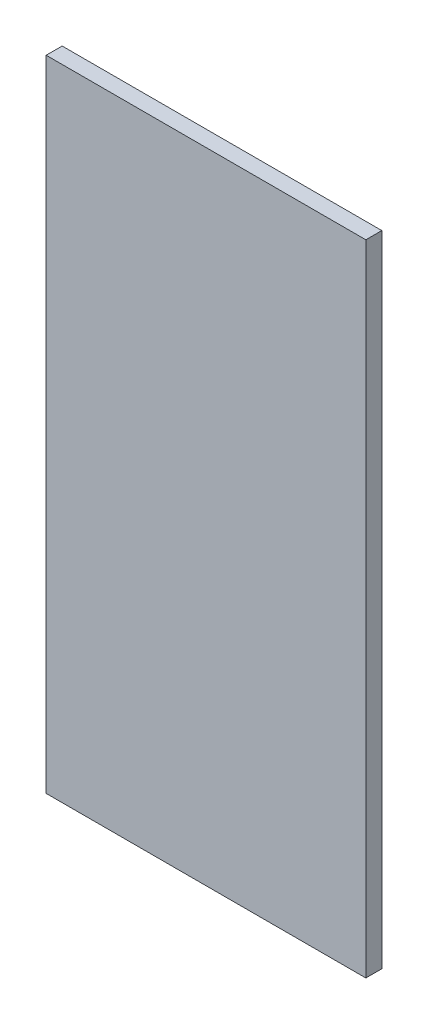
from build123d import *

# Parameters (mm, degrees)
SKETCH1_W           = 600
SKETCH1_H           = 1200
BOSS_EXTRUDE1_DEPTH = 30
SKETCH2_R           = 60
CUT_EXTRUDE1_DEPTH  = 2


with BuildPart() as part:
    # Sketch1 → Boss-Extrude1 (new body)
    with BuildSketch(Plane.XY):
        Rectangle(SKETCH1_W, SKETCH1_H)
    extrude(amount=BOSS_EXTRUDE1_DEPTH)

    # Sketch2 → Cut-Extrude1 (cut)
    with BuildSketch(Plane(origin=(0, 0, 0), x_dir=(-1, 0, 0), z_dir=(0, 0, -1))):
        with Locations((-180, 480)):
            Circle(SKETCH2_R)
        with Locations(Location((180, 480, 0), (0, 0, 180))):
            Circle(SKETCH2_R)
        with Locations((180, -480)):
            Circle(SKETCH2_R)
        with Locations(Location((-180, -480, 0), (0, 0, 180))):
            Circle(SKETCH2_R)
    extrude(amount=-CUT_EXTRUDE1_DEPTH, mode=Mode.SUBTRACT)


solid = part.part
